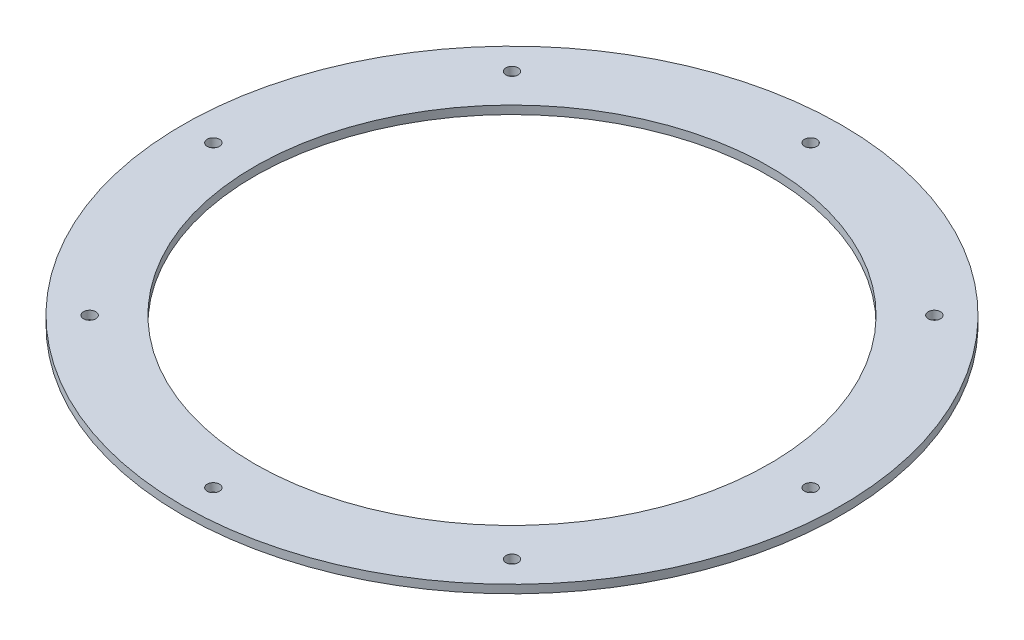
from build123d import *

# Parameters (mm, degrees)
SKETCH_1_R               = 160
SKETCH_1_R_2             = 125
EXTRUDE_1_DEPTH          = 4
SKETCH_2_R               = 3
CUT_EXTRUDE_1_DEPTH      = 227.309522557
PATTERN_CIRCULAR_1_COUNT = 8


with BuildPart() as part:
    # 草图1 → 凸台-拉伸1 (new body)
    with BuildSketch(Plane(origin=(0, 0, 0), x_dir=(1, 0, 0), z_dir=(0, 1, 0))):
        with Locations(Location((0, 0, 0), (0, 0, 270))):
            Circle(SKETCH_1_R)
        with Locations(Location((0, 0, 0), (0, 0, 270))):
            Circle(SKETCH_1_R_2, mode=Mode.SUBTRACT)
    extrude(amount=EXTRUDE_1_DEPTH)

    # 草图2 → 切除-拉伸1 (cut, through all)
    with BuildSketch(Plane(origin=(0, 4, 0), x_dir=(1, 0, 0), z_dir=(0, 1, 0))):
        with Locations(Location((0, 145, 0), (0, 0, 270))):
            Circle(SKETCH_2_R)
    cut_extrude_1 = extrude(amount=-CUT_EXTRUDE_1_DEPTH, mode=Mode.SUBTRACT)

    # 阵列(圆周)1: 切除-拉伸1 ×8 about axis
    pattern_circular_1_axis = Axis((0, 0, 0), (0, 1, 0))
    for i in range(1, PATTERN_CIRCULAR_1_COUNT):
        add(cut_extrude_1.rotate(pattern_circular_1_axis, i * 360 / PATTERN_CIRCULAR_1_COUNT), mode=Mode.SUBTRACT)


solid = part.part
